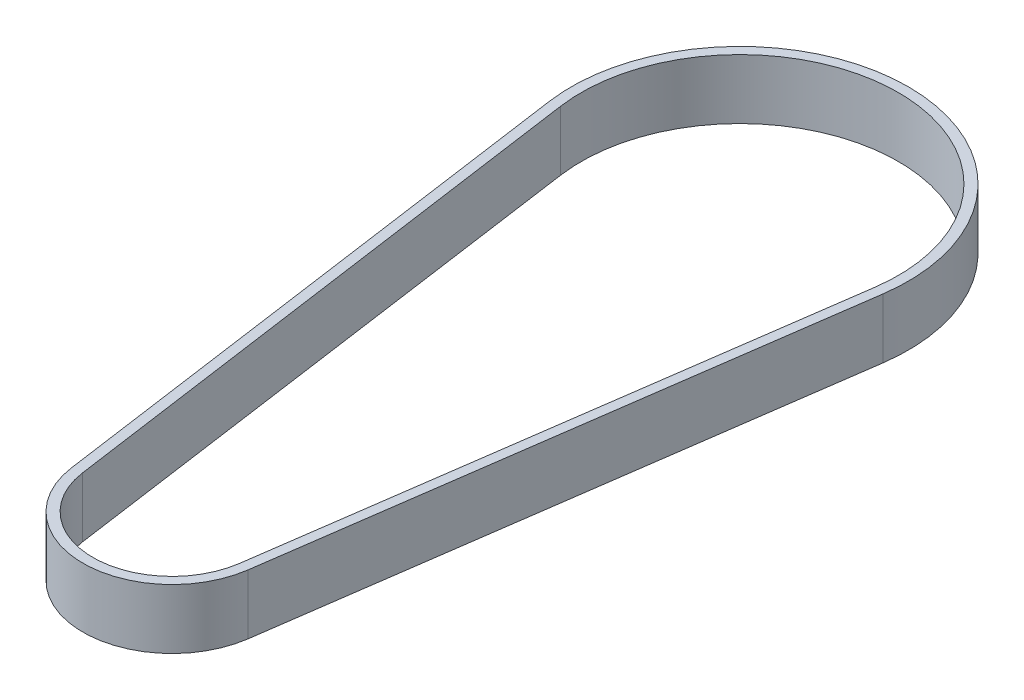
from build123d import *

# Parameters (mm, degrees)
BOSS_EXTRUDE1_DEPTH = 6


with BuildPart() as part:
    # Sketch1 → Boss-Extrude1 (new body)
    with BuildSketch(Plane(origin=(0, 0, 0), x_dir=(1, 0, 0), z_dir=(0, 1, 0))):
        with BuildLine():
            Line((-16.748260586, 54.637974737), (-8.866260216, -1.250418246))
            ThreePointArc((-8.866260216, -1.250418246), (0, -8.954), (8.866260216, -1.250418246))
            Line((8.866260216, -1.250418246), (16.748260586, 54.637974737))
            ThreePointArc((16.748260586, 54.637974737), (0, 73.914), (-16.748260586, 54.637974737))
        make_face()
        with BuildLine():
            Line((-15.758059534, 54.77762386), (-7.876059164, -1.110769123))
            ThreePointArc((-7.876059164, -1.110769123), (0, -7.954), (7.876059164, -1.110769123))
            Line((7.876059164, -1.110769123), (15.758059534, 54.77762386))
            ThreePointArc((15.758059534, 54.77762386), (0, 72.914), (-15.758059534, 54.77762386))
        make_face(mode=Mode.SUBTRACT)
    extrude(amount=BOSS_EXTRUDE1_DEPTH)


solid = part.part
